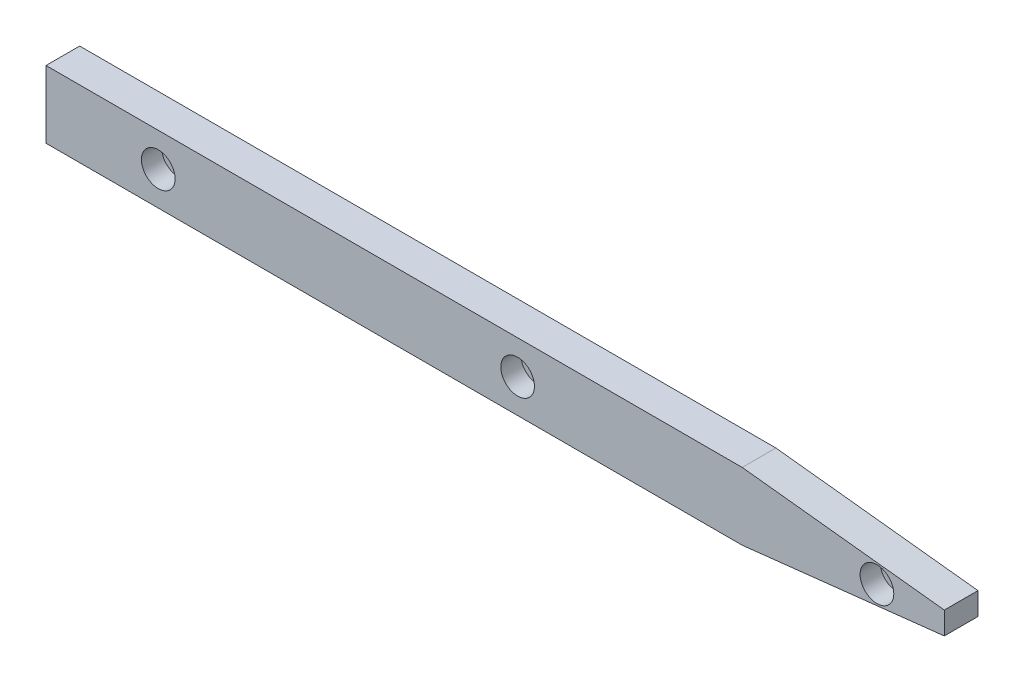
from build123d import *

# Parameters (mm, degrees)
EXTRUDE_1_DEPTH           = 7.5
HOLE_WIZARD_M8_1_D        = 6.8
HOLE_WIZARD_M8_1_DEPTH    = 19.75
HOLE_WIZARD_M8_1_TIP      = 2.042926105
HOLE_WIZARD_1_D           = 9
HOLE_WIZARD_1_CBORE_D     = 15
HOLE_WIZARD_1_CBORE_DEPTH = 9


with BuildPart() as part:
    # 草图1 → 凸台-拉伸1 (new, symmetric)
    with BuildSketch(Plane.XY):
        Polygon((200, 5), (110, 15), (-200, 15), (-200, -15), (110, -15), (200, -5), align=None)
    extrude(amount=EXTRUDE_1_DEPTH, both=True)

    # M8 螺纹孔1
    with Locations(Plane(origin=(-200, 0, 0), x_dir=(0, 0, -1), z_dir=(-1, 0, 0))):
        with Locations((0, 0)):
            Hole(HOLE_WIZARD_M8_1_D / 2, depth=HOLE_WIZARD_M8_1_DEPTH)
            with Locations((0, 0, -(HOLE_WIZARD_M8_1_DEPTH + HOLE_WIZARD_M8_1_TIP / 2))):  # 118° drill point
                Cone(0, HOLE_WIZARD_M8_1_D / 2, HOLE_WIZARD_M8_1_TIP, mode=Mode.SUBTRACT)

    # 打孔尺寸(%根据)内六角圆柱头螺钉的类型1 (through all)
    with Locations(Plane(origin=(-150, 0, 7.5), x_dir=(1, 0, 0), z_dir=(0, 0, 1))):
        with Locations((0, 0), (320, 0), (160, 0)):
            CounterBoreHole(HOLE_WIZARD_1_D / 2, HOLE_WIZARD_1_CBORE_D / 2, HOLE_WIZARD_1_CBORE_DEPTH)


solid = part.part
